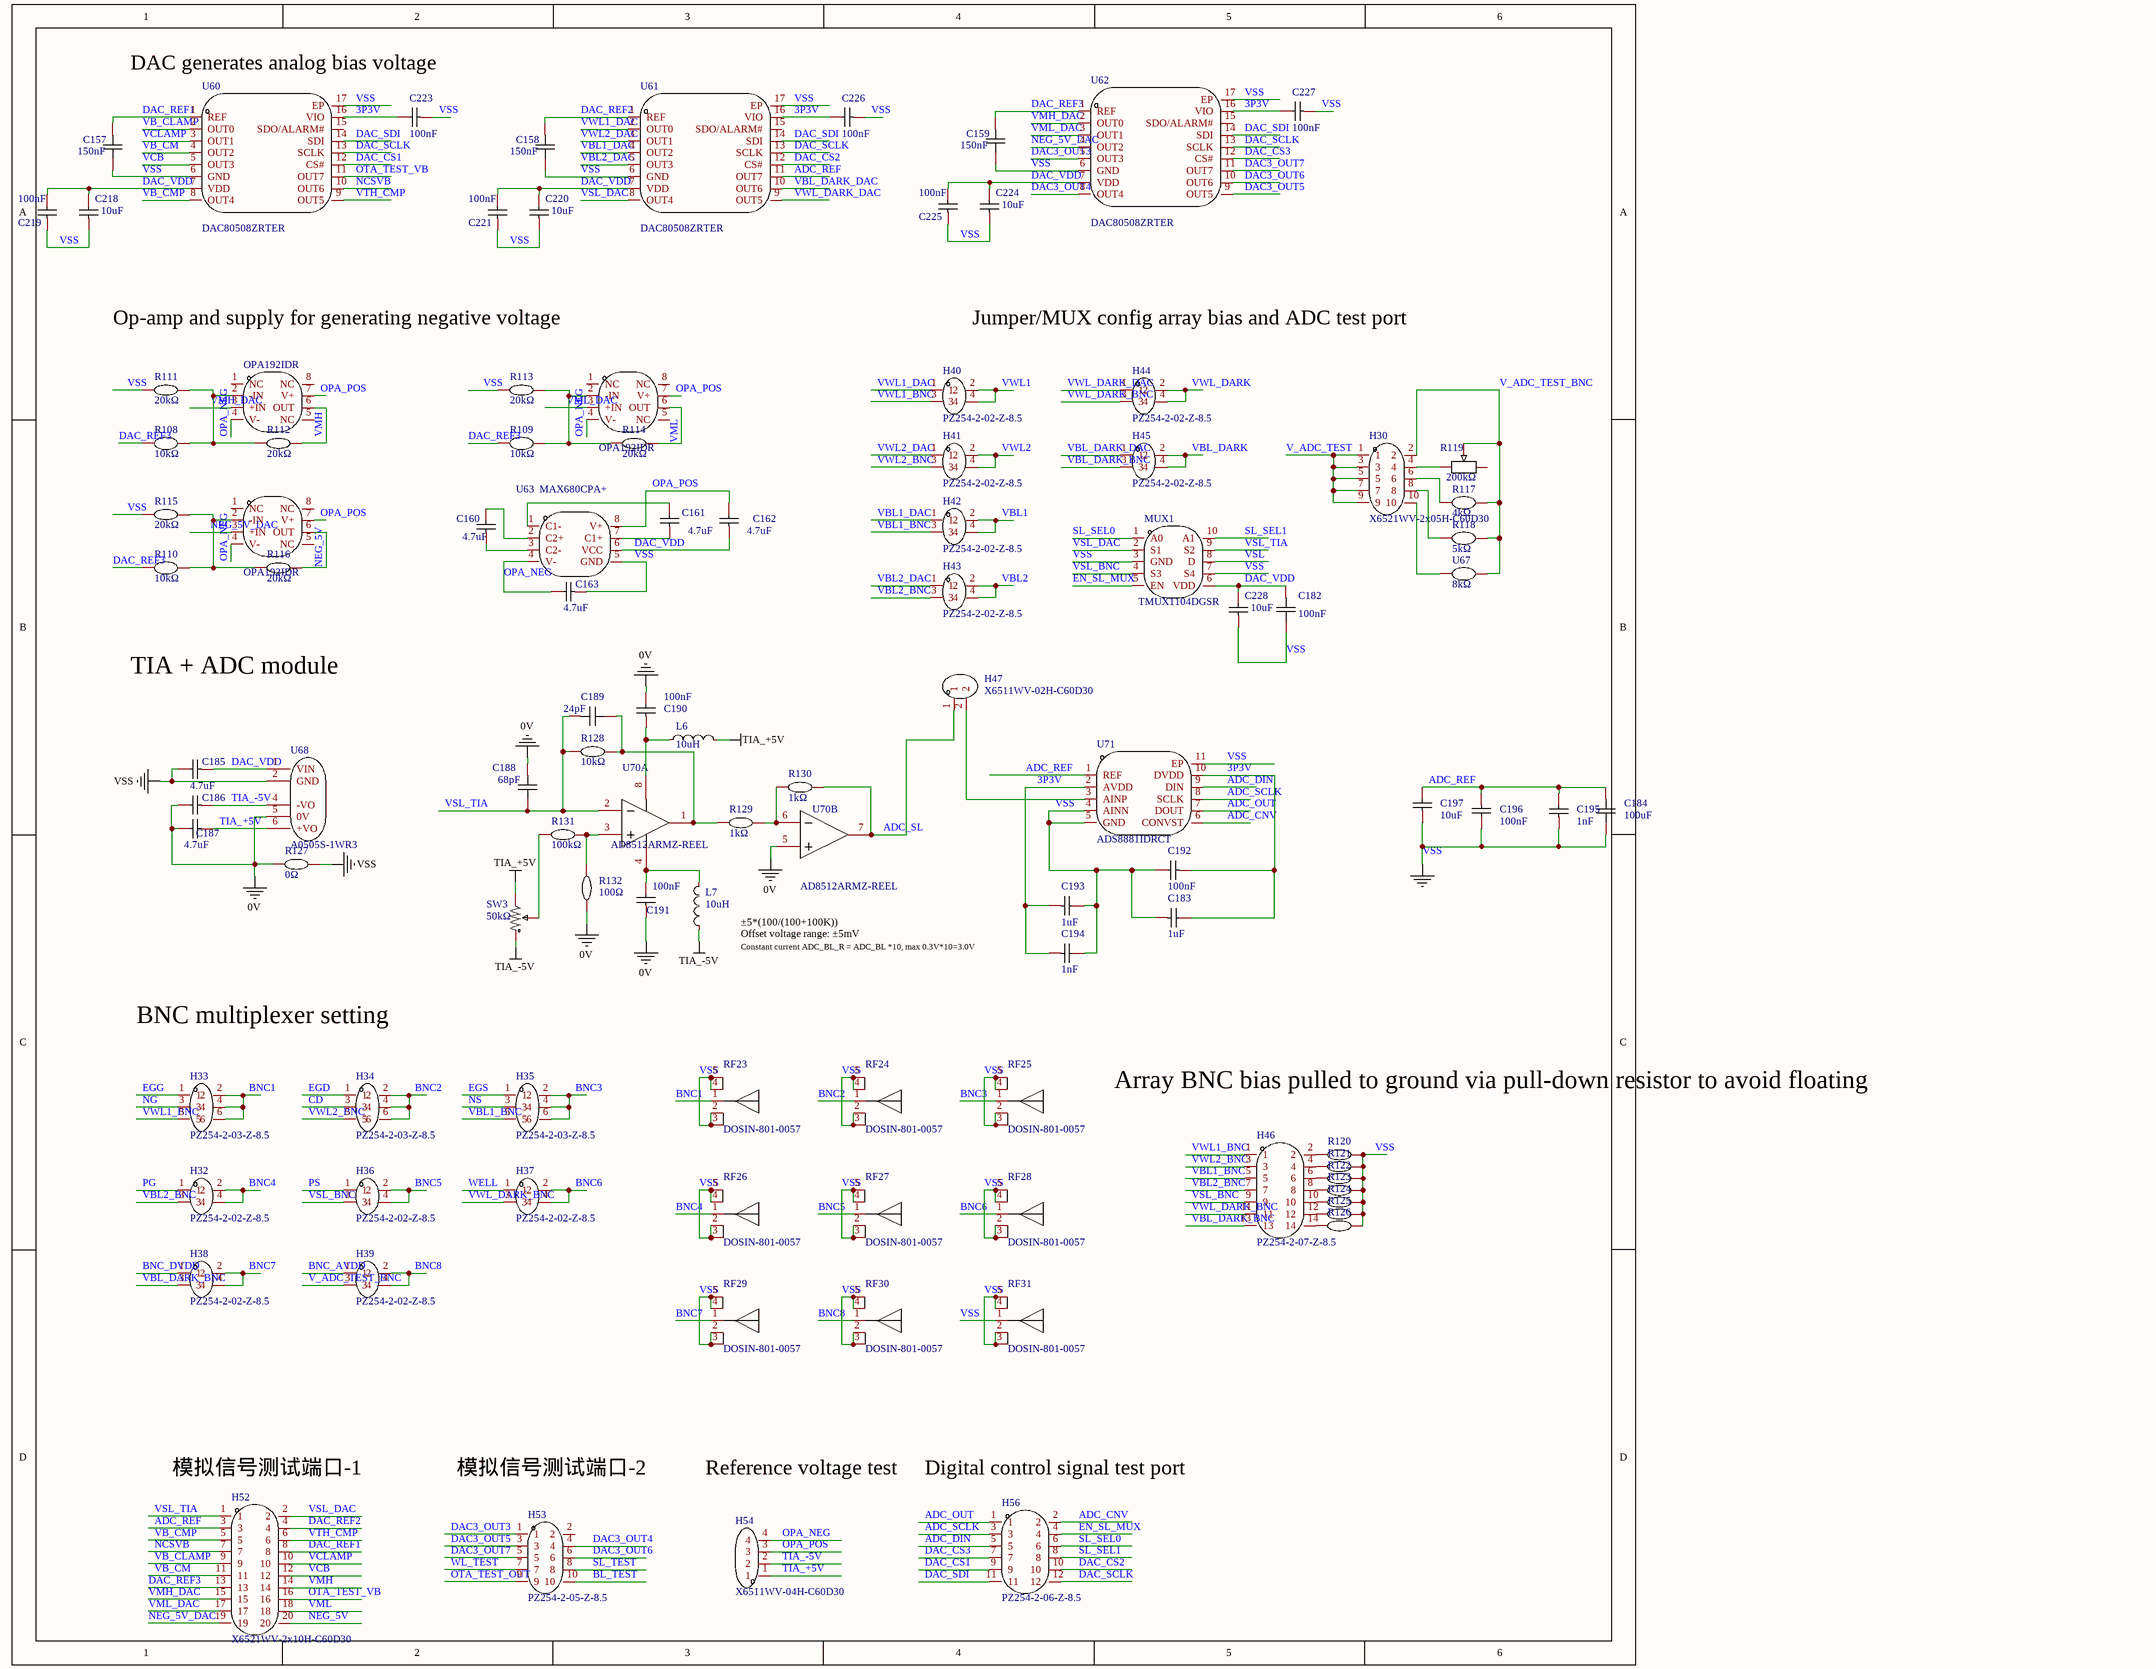
[diagram p0: MISC62793-4.schdoc]
# Altium project MISC62793-14.PrjPcb (part 2 of 4)

## Sheet MISC62793-4.schdoc
size 347 x 355 mm; SheetNumber: 2; SheetTotal: 4

### Parts
C157  150nF  [C0402]
C158  150nF  [C0402]
C159  150nF  [C0402]
C160  4.7uF  [C0805]
C161  4.7uF  [C0805]
C162  4.7uF  [C0805]
C163  4.7uF  [C0805]
C182  100nF  [C0402]
C183  1uF  [C0603]
C184  100uF  [C1210]
C185  4.7uF  [C0805]
C186  4.7uF  [C0805]  (value not drawn)
C187  4.7uF  [C0805]
C188  68pF  [C0402]
C189  24pF  [C0402]
C190  100nF  [C0402]
C191  100nF  [C0402]
C192  100nF  [C0402]
C193  1uF  [C0603]
C194  1nF  [C0603]
C195  1nF  [C0603]
C196  100nF  [C0402]
C197  10uF  [C0805]
C218  10uF  [C0805]
C219  100nF  [C0402]
C220  10uF  [C0805]
C221  100nF  [C0402]
C223  100nF  [C0402]
C224  10uF  [C0805]
C225  100nF  [C0402]
C226  100nF  [C0402]
C227  100nF  [C0402]
C228  10uF  [C0805]
H30  X6521WV-2x05H-C60D30  [HDR-TH_10P-P2.54-V-M-R2-C5-S2.54]
H32  PZ254-2-02-Z-8.5  [HDR-TH_4P-P2.54-V-M-R2-C2-S2.54]
H33  PZ254-2-03-Z-8.5  [HDR-TH_6P-P2.54-V-M-R2-C3-S2.54]
H34  PZ254-2-03-Z-8.5  [HDR-TH_6P-P2.54-V-M-R2-C3-S2.54]
H35  PZ254-2-03-Z-8.5  [HDR-TH_6P-P2.54-V-M-R2-C3-S2.54]
H36  PZ254-2-02-Z-8.5  [HDR-TH_4P-P2.54-V-M-R2-C2-S2.54]
H37  PZ254-2-02-Z-8.5  [HDR-TH_4P-P2.54-V-M-R2-C2-S2.54]
H38  PZ254-2-02-Z-8.5  [HDR-TH_4P-P2.54-V-M-R2-C2-S2.54]
H39  PZ254-2-02-Z-8.5  [HDR-TH_4P-P2.54-V-M-R2-C2-S2.54]
H40  PZ254-2-02-Z-8.5  [HDR-TH_4P-P2.54-V-M-R2-C2-S2.54]
H41  PZ254-2-02-Z-8.5  [HDR-TH_4P-P2.54-V-M-R2-C2-S2.54]
H42  PZ254-2-02-Z-8.5  [HDR-TH_4P-P2.54-V-M-R2-C2-S2.54]
H43  PZ254-2-02-Z-8.5  [HDR-TH_4P-P2.54-V-M-R2-C2-S2.54]
H44  PZ254-2-02-Z-8.5  [HDR-TH_4P-P2.54-V-M-R2-C2-S2.54]
H45  PZ254-2-02-Z-8.5  [HDR-TH_4P-P2.54-V-M-R2-C2-S2.54]
H46  PZ254-2-07-Z-8.5  [HDR-TH_14P-P2.54-V-M-R2-C7-S2.54]
H47  X6511WV-02H-C60D30  [HDR-TH_2P-P2.54-V-M]
H52  X6521WV-2x10H-C60D30  [HDR-TH_20P-P2.54-V-M-R2-C10-S2.54]
H53  PZ254-2-05-Z-8.5  [HDR-TH_10P-P2.54-V-M-R2-C5-S2.54]
H54  X6511WV-04H-C60D30  [HDR-TH_4P-P2.54-V-M]
H56  PZ254-2-06-Z-8.5  [HDR-TH_12P-P2.54-V-M-R2-C6-S2.54]
L6  10uH  [IND-SMD_L7.3-W6.8]
L7  10uH  [IND-SMD_L7.3-W6.8]
MUX1  TMUX1104DGSR  [VSSOP-10_L3.0-W3.0-P0.50-LS4.9-BL]
R108  10kΩ  [R0603]
R109  10kΩ  [R0603]
R110  10kΩ  [R0603]
R111  20kΩ  [R0805]
R112  20kΩ  [R0805]
R113  20kΩ  [R0805]
R114  20kΩ  [R0805]
R115  20kΩ  [R0805]
R116  20kΩ  [R0805]
R117  4kΩ  [R0805]
R118  5kΩ  [R0805]
R119  200kΩ  [RES-ADJ-SMD_3P-L4.5-W4.5-P2.30-BL-FS]
R120  1MΩ  [R1206]  (value not drawn)
R121  1MΩ  [R1206]  (value not drawn)
R122  1MΩ  [R1206]  (value not drawn)
R123  1MΩ  [R1206]  (value not drawn)
R124  1MΩ  [R1206]  (value not drawn)
R125  1MΩ  [R1206]  (value not drawn)
R126  1MΩ  [R1206]  (value not drawn)
R127  0Ω  [R0603]
R128  10kΩ  [R0603]
R129  1kΩ  [R0805]
R130  1kΩ  [R0805]
R131  100kΩ  [R0603]
R132  100Ω  [R1206]
RF23  DOSIN-801-0057  [ANT-TH_DOSIN-801-0057]
RF24  DOSIN-801-0057  [ANT-TH_DOSIN-801-0057]
RF25  DOSIN-801-0057  [ANT-TH_DOSIN-801-0057]
RF26  DOSIN-801-0057  [ANT-TH_DOSIN-801-0057]
RF27  DOSIN-801-0057  [ANT-TH_DOSIN-801-0057]
RF28  DOSIN-801-0057  [ANT-TH_DOSIN-801-0057]
RF29  DOSIN-801-0057  [ANT-TH_DOSIN-801-0057]
RF30  DOSIN-801-0057  [ANT-TH_DOSIN-801-0057]
RF31  DOSIN-801-0057  [ANT-TH_DOSIN-801-0057]
SW3  50kΩ  [RES-ADJ-SMD_3P-L6.0-W4.3-P5.00-BL]
U60  DAC80508ZRTER  [WQFN-16_L3.0-W3.0-P0.50-TL-EP0.8]
U61  DAC80508ZRTER  [WQFN-16_L3.0-W3.0-P0.50-TL-EP0.8]
U62  DAC80508ZRTER  [WQFN-16_L3.0-W3.0-P0.50-TL-EP0.8]
U63  MAX680CPA+  [DIP-8_L10.1-W6.3-P2.54-LS7.6-BL]
U64  OPA192IDR  [SOIC-8_L4.9-W3.9-P1.27-LS6.0-BL]
U65  OPA192IDR  [SOIC-8_L4.9-W3.9-P1.27-LS6.0-BL]
U66  OPA192IDR  [SOIC-8_L4.9-W3.9-P1.27-LS6.0-BL]
U67  8kΩ  [R0805]
U68  A0505S-1WR3  [PWRM-TH_A05XXS-1WR3]
U70  AD8512ARMZ-REEL  [MSOP-8_L3.0-W3.0-P0.65-LS5.0-TL]  (parts A,B of 2)
U71  ADS8881IDRCT  [VSON-10_L3.0-W3.0-P0.50-TL-EP-3]

### Nets
0V: C186.2 C187.2 C188.2 C190.2 C191.1 R127.1 R132.1 U68.5(0V) U70.5(+IN_B)
TIA_+5V: C187.1 H54.1 L6.2 SW3.3 U68.6(+VO)
TIA_-5V: C186.1 H54.2 L7.1 SW3.1 U68.4(-VO)
VSS: C157.1 C158.1 C159.1 C163.1 C182.1 C183.1 C184.1 C185.2 C192.2 C193.2 C194.2 C195.1 C196.2 C197.1 C218.1 C219.1 C220.1 C221.1 C223.1 C224.1 C225.1 C226.1 C227.1 C228.1 MUX1.3(GND) MUX1.7(S4) R111.1 R113.1 R115.1 R120.2 R121.2 R122.2 R123.2 R124.2 R125.2 R126.2 R127.2 RF23.2 RF23.3 RF23.4 RF23.5 RF24.2 RF24.3 RF24.4 RF24.5 RF25.2 RF25.3 RF25.4 RF25.5 RF26.2 RF26.3 RF26.4 RF26.5 RF27.2 RF27.3 RF27.4 RF27.5 RF28.2 RF28.3 RF28.4 RF28.5 RF29.2 RF29.3 RF29.4 RF29.5 RF30.2 RF30.3 RF30.4 RF30.5 RF31.1 RF31.2 RF31.3 RF31.4 RF31.5 U60.6(GND) U60.17(EP) U61.6(GND) U61.17(EP) U62.6(GND) U62.17(EP) U63.5(GND) U68.2(GND) U71.4(AINN) U71.5(GND) U71.11(EP)
3P3V: C183.2 C192.1 C193.1 C194.1 C223.2 C226.2 C227.2 U60.16(VIO) U61.16(VIO) U62.16(VIO) U71.2(AVDD) U71.10(DVDD)
ADC_CNV: H56.2 U71.6(CONVST)
ADC_DIN: H56.5 U71.9(DIN)
ADC_OUT: H56.1 U71.7(DOUT)
ADC_REF: C184.2 C195.2 C196.1 C197.2 H52.3 U61.11(OUT7) U71.1(REF)
ADC_SCLK: H56.3 U71.8(SCLK)
ADC_SL: H47.1 R130.2 U70.7(OUT_B)
BL_TEST: H53.10
BNC1: H33.2 H33.4 H33.6 RF23.1
BNC2: H34.2 H34.4 H34.6 RF24.1
BNC3: H35.2 H35.4 H35.6 RF25.1
BNC4: H32.2 H32.4 RF26.1
BNC5: H36.2 H36.4 RF27.1
BNC6: H37.2 H37.4 RF28.1
BNC7: H38.2 H38.4 RF29.1
BNC8: H39.2 H39.4 RF30.1
BNC_AVDD: H39.1
BNC_DVDD: H38.1
CD: H34.3
DAC3_OUT3: H53.1 U62.5(OUT3)
DAC3_OUT4: H53.4 U62.8(OUT4)
DAC3_OUT5: H53.3 U62.9(OUT5)
DAC3_OUT6: H53.6 U62.10(OUT6)
DAC3_OUT7: H53.5 U62.11(OUT7)
DAC_CS1: H56.9 U60.12(CS#)
DAC_CS2: H56.10 U61.12(CS#)
DAC_CS3: H56.7 U62.12(CS#)
DAC_REF1: C157.2 H52.8 U60.1(REF)
DAC_REF2: C158.2 H52.4 U61.1(REF)
DAC_REF3: C159.2 H52.13 R108.1 R109.1 R110.1 U62.1(REF)
DAC_SCLK: H56.12 U60.13(SCLK) U61.13(SCLK) U62.13(SCLK)
DAC_SDI: H56.11 U60.14(SDI) U61.14(SDI) U62.14(SDI)
DAC_VDD: C162.1 C182.2 C185.1 C218.2 C219.2 C220.2 C221.2 C224.2 C225.2 C228.2 MUX1.6(VDD) U60.7(VDD) U61.7(VDD) U62.7(VDD) U63.6(VCC) U68.1(VIN)
EGD: H34.1
EGG: H33.1
EGS: H35.1
EN_SL_MUX: H56.4 MUX1.5(EN)
NCSVB: H52.7 U60.10(OUT6)
NEG_5V: H52.20 R116.2 U65.6(OUT)
NEG_5V_DAC: H52.19 U62.4(OUT2) U65.3(+IN)
NG: H33.3
NS: H35.3
OPA_NEG: C163.2 H54.4 U63.4(V-) U64.4(V-) U65.4(V-) U66.4(V-)
OPA_POS: C162.2 H54.3 U63.8(V+) U64.7(V+) U65.7(V+) U66.7(V+)
OTA_TEST_OUT: H53.9
OTA_TEST_VB: H52.16 U60.11(OUT7)
PG: H32.1
PS: H36.1
SL_SEL0: H56.6 MUX1.1(A0)
SL_SEL1: H56.8 MUX1.10(A1)
SL_TEST: H53.8
V_ADC_TEST: H30.1 H30.3 H30.5 H30.7 H30.9
V_ADC_TEST_BNC: H30.2 H39.3 R117.2 R118.2 R119.2 U67.2
VB_CLAMP: H52.9 U60.2(OUT0)
VB_CM: H52.11 U60.4(OUT2)
VB_CMP: H52.5 U60.8(OUT4)
VBL1: H42.2 H42.4
VBL1_BNC: H35.5 H42.3 H46.5
VBL1_DAC: H42.1 U61.4(OUT2)
VBL2: H43.2 H43.4
VBL2_BNC: H32.3 H43.3 H46.7
VBL2_DAC: H43.1 U61.5(OUT3)
VBL_DARK: H45.2 H45.4
VBL_DARK_BNC: H38.3 H45.3 H46.13
VBL_DARK_DAC: H45.1 U61.10(OUT6)
VCB: H52.12 U60.5(OUT3)
VCLAMP: H52.10 U60.3(OUT1)
VMH: H52.14 R112.2 U64.6(OUT)
VMH_DAC: H52.15 U62.2(OUT0) U64.3(+IN)
VML: H52.18 R114.2 U66.6(OUT)
VML_DAC: H52.17 U62.3(OUT1) U66.3(+IN)
VSL: MUX1.8(D)
VSL_BNC: H36.3 H46.9 MUX1.4(S3)
VSL_DAC: H52.2 MUX1.2(S1) U61.8(OUT4)
VSL_TIA: C188.1 C189.2 H52.1 MUX1.9(S2) R128.1 U70.2(-IN_A)
VTH_CMP: H52.6 U60.9(OUT5)
VWL1: H40.2 H40.4
VWL1_BNC: H33.5 H40.3 H46.1
VWL1_DAC: H40.1 U61.2(OUT0)
VWL2: H41.2 H41.4
VWL2_BNC: H34.5 H41.3 H46.3
VWL2_DAC: H41.1 U61.3(OUT1)
VWL_DARK: H44.2 H44.4
VWL_DARK_BNC: H37.3 H44.3 H46.11
VWL_DARK_DAC: H44.1 U61.9(OUT5)
WELL: H37.1
WL_TEST: H53.7
NetC160_1: C160.1 U63.3(C2-)
NetC160_2: C160.2 U63.2(C2+)
NetC161_1: C161.1 U63.7(C1+)
NetC161_2: C161.2 U63.1(C1-)
NetC189_1: C189.1 R128.2 R129.1 U70.1(OUT_A)
NetC190_1: C190.1 L6.1 U70.8(V+)
NetC191_2: C191.2 L7.2 U70.4(V-)
NetH30_4: H30.4 R119.1
NetH30_6: H30.6 R117.1
NetH30_8: H30.8 R118.1
NetH30_10: H30.10 U67.1
NetH46_2: H46.2 R120.1
NetH46_4: H46.4 R121.1
NetH46_6: H46.6 R122.1
NetH46_8: H46.8 R123.1
NetH46_10: H46.10 R124.1
NetH46_12: H46.12 R125.1
NetH46_14: H46.14 R126.1
NetH47_2: H47.2 U71.3(AINP)
NetR108_2: R108.2 R111.2 R112.1 U64.2(-IN)
NetR109_2: R109.2 R113.2 R114.1 U66.2(-IN)
NetR110_2: R110.2 R115.2 R116.1 U65.2(-IN)
NetR129_2: R129.2 R130.1 U70.6(-IN_B)
NetR131_1: R131.1 SW3.2
NetR131_2: R131.2 R132.2 U70.3(+IN_A)

Not connected (* = marked no-connect by the designer): H53 2; R119 3; U60 15(SDO/ALARM#); U61 15(SDO/ALARM#); U62 15(SDO/ALARM#); U64 1(NC) 5(NC) 8(NC); U65 1(NC) 5(NC) 8(NC); U66 1(NC) 5(NC) 8(NC)

### Notes on the sheet
- DAC generates analog bias voltage
- Op-amp and supply for generating negative voltage
- Jumper/MUX config array bias and ADC test port
- TIA + ADC module
- (near L7) Offset voltage range: ±5mV
- (near L7) ±5*(100/(100+100K))
- (near L7) Constant current ADC_BL_R = ADC_BL *10, max 0.3V*10=3.0V
- BNC multiplexer setting
- Array BNC bias pulled to ground via pull-down resistor to avoid floating
- (near H52) 模拟信号测试端口-1
- 模拟信号测试端口-2
- Reference voltage test
- (near H56) Digital control signal test port

### Library data of the parts
C157-C159 = CC0402KRX5R7BB154: Manufacturer: YAGEO(国巨); Add into BOM: yes; Tolerance: ±10%; Voltage Rated: 16V; Temperature Coefficient: X5R; Name: 150nF; Symbol: CC0402KRX5R7BB154; Device: CC0402KRX5R7BB154; Supplier: LCSC; Supplier Part: C576725; Manufacturer Part: CC0402KRX5R7BB154; Value: 150nF; JLCPCB Part Class: JLCPCB Part Class: Extended library; LCSC Part Name: 150nF ±10% 16V; Supplier Footprint: 0402; Datasheet: https://example.com/upload/public/pdf/source/20200331/C505498_E84D0E375B576359B11079CF792A6AF0.pdf; Convert to PCB: yes
C160-C163 C185-C187 = CL21A475KBQNNNE: Manufacturer: SAMSUNG(三星); Add into BOM: yes; Tolerance: ±10%; Voltage Rated: 50V; Temperature Coefficient: X5R; Name: 4.7uF; Symbol: CL21A475KBQNNNE; Device: CL21A475KBQNNNE; LCSC Part Name: 4.7uF ±10% 50V; Supplier Part: C98192; Manufacturer Part: CL21A475KBQNNNE; Supplier Footprint: 0805; JLCPCB Part Class: JLCPCB Part Class: Extended library; Datasheet: https://example.com/upload/public/pdf/source/20160218/1457707763339.pdf; Supplier: LCSC; Convert to PCB: yes; Value: 4.7uF
C182 = CC0402KRX7R7BB104: Manufacturer: YAGEO(国巨); Add into BOM: yes; Tolerance: ±10%; Voltage Rated: 16V; Temperature Coefficient: X7R; Name: 100nF; Symbol: CC0402KRX7R7BB104; Device: CC0402KRX7R7BB104; Supplier: LCSC; Manufacturer Part: CC0402KRX7R7BB104; Value: 100nF; Supplier Part: C60474; JLCPCB Part Class: JLCPCB Part Class: Extended library; LCSC Part Name: 100nF ±10% 16V; Supplier Footprint: 0402; Datasheet: https://example.com/upload/public/pdf/source/20211223/9278FD768280B81DDBEF48FA36411A03.pdf; Convert to PCB: yes
C183 C193 = CL10A105KO8NNNC: Manufacturer: SAMSUNG(三星); Add into BOM: yes; Tolerance: ±10%; Voltage Rated: 16V; Temperature Coefficient: X5R; Name: 1uF; Symbol: CL10A105KO8NNNC; Device: CL10A105KO8NNNC; LCSC Part Name: 1uF ±10% 16V; Supplier Part: C1592; Manufacturer Part: CL10A105KO8NNNC; Supplier Footprint: 0603; JLCPCB Part Class: JLCPCB Part Class: Extended library; Datasheet: https://example.com/upload/public/pdf/source/20220919/9FBE606BE0D9532D730F292EB26DC5BB.pdf; Supplier: LCSC; Convert to PCB: yes; Value: 1uF
C184 = EMK325ABJ107MM-P: Manufacturer: TAIYO YUDEN(太诱); Add into BOM: yes; Tolerance: ±20%; Voltage Rated: 16V; Temperature Coefficient: X5R; Name: 100uF; Symbol: EMK325ABJ107MM-P; Device: EMK325ABJ107MM-P; Supplier: LCSC; Supplier Part: C90143; Manufacturer Part: EMK325ABJ107MM-P; Value: 100uF; JLCPCB Part Class: JLCPCB Part Class: Extended library; LCSC Part Name: 100uF ±20% 16V; Supplier Footprint: 1210; Datasheet: https://example.com/upload/public/pdf/source/20190902/C90143_6CB75A095DFF9740D13406046689E055.pdf; Convert to PCB: yes
C188 = CC0402FRNPO9BN680: Manufacturer: YAGEO(国巨); Add into BOM: yes; Tolerance: ±1%; Voltage Rated: 50V; Temperature Coefficient: NP0; Name: 68pF; Symbol: CC0402FRNPO9BN680; Device: CC0402FRNPO9BN680; Supplier: LCSC; Supplier Part: C389103; Manufacturer Part: CC0402FRNPO9BN680; Value: 68pF; JLCPCB Part Class: JLCPCB Part Class: Extended library; LCSC Part Name: 68pF ±1% 50V; Supplier Footprint: 0402; Datasheet: https://example.com/upload/public/pdf/source/20190423/C389103_68497E1D404C7FF179120BC230675ADA.pdf; Convert to PCB: yes
C189 = GJM1555C1H240FB01D: Manufacturer: muRata(村田); Add into BOM: yes; Tolerance: ±1%; Voltage Rated: 50V; Temperature Coefficient: C0G; Name: 24pF; Symbol: GJM1555C1H240FB01D; Device: GJM1555C1H240FB01D; Supplier: LCSC; Supplier Part: C415394; Manufacturer Part: GJM1555C1H240FB01D; Value: 24pF; JLCPCB Part Class: JLCPCB Part Class: Extended library; LCSC Part Name: 24pF ±1% 50V; Supplier Footprint: 0402; Datasheet: https://example.com/upload/public/pdf/source/20190904/C426118_85E81C7C1F21FC87C5FB6D536E0847B4.pdf; Convert to PCB: yes
C190-C192 C196 C219 C221 C223 C225-C227 = CL05B104KO5NNNC: Manufacturer: SAMSUNG(三星); Add into BOM: yes; Tolerance: ±10%; Voltage Rated: 16V; Temperature Coefficient: X7R; Name: 100nF; Symbol: CL05B104KO5NNNC; Device: CL05B104KO5NNNC; Supplier: LCSC; Manufacturer Part: CL05B104KO5NNNC; Value: 100nF; Supplier Part: C1525; JLCPCB Part Class: JLCPCB Part Class: Basic library; LCSC Part Name: 100nF ±10% 16V; Supplier Footprint: 0402; Datasheet: https://example.com/upload/public/pdf/source/20160218/1457707763339.pdf; Convert to PCB: yes
C194 C195 = CC0603KRX7R9BB102: Manufacturer: YAGEO(国巨); Add into BOM: yes; Tolerance: ±10%; Voltage Rated: 50V; Temperature Coefficient: X7R; Name: 1nF; Symbol: CC0603KRX7R9BB102; Device: CC0603KRX7R9BB102; Supplier: LCSC; Manufacturer Part: CC0603KRX7R9BB102; Value: 1nF; Supplier Part: C100040; JLCPCB Part Class: JLCPCB Part Class: Extended library; LCSC Part Name: 1nF ±10% 50V; Supplier Footprint: 0603; Datasheet: https://example.com/upload/public/pdf/source/20180910/C282072_33301C7F631E79921B82A8DAC6BCC5B3.pdf; Convert to PCB: yes
C197 C218 C220 C224 C228 = CL21A106KOQNNNE: Manufacturer: SAMSUNG(三星); Add into BOM: yes; Tolerance: ±10%; Voltage Rated: 16V; Temperature Coefficient: X5R; Name: 10uF; Symbol: CL21A106KOQNNNE; Device: CL21A106KOQNNNE; Supplier: LCSC; Manufacturer Part: CL21A106KOQNNNE; Value: 10uF; Supplier Part: C1713; JLCPCB Part Class: JLCPCB Part Class: Extended library; LCSC Part Name: 10uF ±10% 16V; Supplier Footprint: 0805; Datasheet: https://example.com/upload/public/pdf/source/20160218/1457707763339.pdf; Convert to PCB: yes
H30 = X6521WV-2x05H-C60D30: Manufacturer: XKB Connection(中国星坤); Symbol: X6521WV-2×05H-C30D60; Add into BOM: yes; Pin Structure: 2x5P; Pitch: 2.54mm; Circluar Pins/Square Pins: Square pin; Current Rating (Max): 3A; Voltage Rating (Max): 250V; Soldering Temperature(Max): 260℃; Name: X6521WV-2x05H-C60D30; Device: X6521WV-2x05H-C60D30; LCSC Part Name: 2x5P 间距:2.54mm 方针; Supplier Part: C706895; Manufacturer Part: X6521WV-2x05H-C60D30; Supplier Footprint: 插件,P=2.54mm; JLCPCB Part Class: JLCPCB Part Class: Extended library; Datasheet: https://example.com/upload/public/pdf/source/20211009/DE33EBA4104B5B447A7BD8383FBBA145.pdf; Supplier: LCSC; Convert to PCB: yes; Row Spacing: 2.54mm; Mounting Type: -; Number of Rows: Dual row; Number of Pins: 10P; Length of Mating Pin: 6mm; Insulation Height: 2.5mm; Length of End Connection Pin: 3mm; Contact Material: Brass; Contact Plating: Gold; Operating Temperature Range: -40℃~+105℃; Color: Black
H32 H36-H45 = PZ254-2-02-Z-8.5_C2894963: Manufacturer: HCTL(华灿天禄); Add into BOM: yes; Pin Structure: 2x2P; Pitch: 2.54mm; Circluar Pins/Square Pins: Square pin; Current Rating (Max): 3A; Soldering Temperature(Max): 260℃@10S; Name: PZ254-2-02-Z-8.5; Symbol: PZ254-2-02-Z-8.5; Device: PZ254-2-02-Z-8.5_C2894963; LCSC Part Name: 2x2P 间距:2.54mm 方针 直插; Supplier Part: C2894963; Manufacturer Part: PZ254-2-02-Z-8.5; Supplier Footprint: 插件,P=2.54mm; JLCPCB Part Class: JLCPCB Part Class: Extended library; Datasheet: https://example.com/upload/public/pdf/source/20230609/5BA09C8BEB9B31376F8BF6032FF67CAC.pdf; Supplier: LCSC; Convert to PCB: yes; Row Spacing: 2.54mm; Mounting Type: Through hole; Number of Rows: Dual row; Number of Pins: 4P; Voltage Rating (Max): -; Length of Mating Pin: 6mm; Insulation Height: 2.5mm; Length of End Connection Pin: 3mm; Contact Material: Brass; Operating Temperature Range: -40℃~+105℃; Color: Black
H33-H35 = PZ254-2-03-Z-8.5_C2894964: Manufacturer: HCTL(华灿天禄); Add into BOM: yes; Pin Structure: 2x3P; Pitch: 2.54mm; Circluar Pins/Square Pins: Square pin; Current Rating (Max): 3A; Soldering Temperature(Max): 260℃@10S; Name: PZ254-2-03-Z-8.5; Symbol: PZ254-2-03-Z-8.5; Device: PZ254-2-03-Z-8.5_C2894964; LCSC Part Name: 2x3P 间距:2.54mm 方针 直插; Supplier Part: C2894964; Manufacturer Part: PZ254-2-03-Z-8.5; Supplier Footprint: 插件,P=2.54mm; JLCPCB Part Class: JLCPCB Part Class: Extended library; Datasheet: https://example.com/upload/public/pdf/source/20230609/5BA09C8BEB9B31376F8BF6032FF67CAC.pdf; Supplier: LCSC; Convert to PCB: yes; Row Spacing: 2.54mm; Mounting Type: Through hole; Number of Rows: Dual row; Number of Pins: 6P; Voltage Rating (Max): -; Length of Mating Pin: 6mm; Insulation Height: 2.5mm; Length of End Connection Pin: 3mm; Contact Material: Brass; Operating Temperature Range: -40℃~+105℃; Color: Black
H46 = PZ254-2-07-Z-8.5: Manufacturer: HCTL(华灿天禄); Add into BOM: yes; Pin Structure: 2x7P; Pitch: 2.54mm; Circluar Pins/Square Pins: Square pin; Current Rating (Max): 3A; Soldering Temperature(Max): 260℃@10S; Name: PZ254-2-07-Z-8.5; Symbol: PZ254-2-07-Z-8.5; Device: PZ254-2-07-Z-8.5; LCSC Part Name: 2x7P 间距:2.54mm 方针 直插; Supplier Part: C2894968; Manufacturer Part: PZ254-2-07-Z-8.5; Supplier Footprint: 插件,P=2.54mm; JLCPCB Part Class: JLCPCB Part Class: Extended library; Datasheet: https://example.com/upload/public/pdf/source/20230609/5BA09C8BEB9B31376F8BF6032FF67CAC.pdf; Supplier: LCSC; Convert to PCB: yes; Row Spacing: 2.54mm; Mounting Type: Through hole; Number of Rows: Dual row; Number of Pins: 14P; Voltage Rating (Max): -; Length of Mating Pin: 6mm; Insulation Height: 2.5mm; Length of End Connection Pin: 3mm; Contact Material: Brass; Operating Temperature Range: -40℃~+105℃; Color: Black
H47 = X6511WV-02H-C60D30: Manufacturer: XKB Connection(中国星坤); Symbol: X6511WV-02H-C30D60; Add into BOM: yes; Pin Structure: 1x2P; Pitch: 2.54mm; Circluar Pins/Square Pins: Square pin; Current Rating (Max): 3A; Voltage Rating (Max): 250V; Soldering Temperature(Max): 260℃; Name: X6511WV-02H-C60D30; Device: X6511WV-02H-C60D30; LCSC Part Name: 1x2P 间距:2.54mm 方针; Supplier Part: C706874; Manufacturer Part: X6511WV-02H-C60D30; Supplier Footprint: 插件,P=2.54mm; JLCPCB Part Class: JLCPCB Part Class: Extended library; Supplier: LCSC; Convert to PCB: yes; Row Spacing: 2.54mm; Mounting Type: -; Number of Rows: Single row; Number of Pins: 2P; Length of Mating Pin: 6mm; Insulation Height: 2.5mm; Length of End Connection Pin: 3mm; Contact Material: Brass; Contact Plating: Gold; Operating Temperature Range: -40℃~+105℃; Color: Black
H52 = X6521WV-2x10H-C60D30: Manufacturer: XKB Connection(中国星坤); Symbol: X6521WV-2×10H-C30D60; Add into BOM: yes; Pin Structure: 2x10P; Pitch: 2.54mm; Circluar Pins/Square Pins: Square pin; Current Rating (Max): 3A; Voltage Rating (Max): 250V; Soldering Temperature(Max): 260℃; Name: X6521WV-2x10H-C60D30; Device: X6521WV-2x10H-C60D30; LCSC Part Name: 2x10P 间距:2.54mm 方针; Supplier Part: C706900; Manufacturer Part: X6521WV-2x10H-C60D30; Supplier Footprint: 插件,P=2.54mm; JLCPCB Part Class: JLCPCB Part Class: Extended library; Datasheet: https://example.com/upload/public/pdf/source/20211009/DE33EBA4104B5B447A7BD8383FBBA145.pdf; Supplier: LCSC; Convert to PCB: yes; Row Spacing: 2.54mm; Mounting Type: -; Number of Rows: Dual row; Number of Pins: 20P; Length of Mating Pin: 6mm; Insulation Height: 2.5mm; Length of End Connection Pin: 3mm; Contact Material: Brass; Contact Plating: Gold; Operating Temperature Range: -40℃~+105℃; Color: Black
H53 = PZ254-2-05-Z-8.5_C2894966: Manufacturer: HCTL(华灿天禄); Add into BOM: yes; Pin Structure: 2x5P; Pitch: 2.54mm; Circluar Pins/Square Pins: Square pin; Current Rating (Max): 3A; Soldering Temperature(Max): 260℃@10S; Name: PZ254-2-05-Z-8.5; Symbol: PZ254-2-05-Z-8.5; Device: PZ254-2-05-Z-8.5_C2894966; LCSC Part Name: 2x5P 间距:2.54mm 方针 直插; Supplier Part: C2894966; Manufacturer Part: PZ254-2-05-Z-8.5; Supplier Footprint: 插件,P=2.54mm; JLCPCB Part Class: JLCPCB Part Class: Extended library; Datasheet: https://example.com/upload/public/pdf/source/20230609/5BA09C8BEB9B31376F8BF6032FF67CAC.pdf; Supplier: LCSC; Convert to PCB: yes; Row Spacing: 2.54mm; Mounting Type: Through hole; Number of Rows: Dual row; Number of Pins: 10P; Voltage Rating (Max): -; Length of Mating Pin: 6mm; Insulation Height: 2.5mm; Length of End Connection Pin: 3mm; Contact Material: Brass; Operating Temperature Range: -40℃~+105℃; Color: Black
H54 = X6511WV-04H-C60D30: Manufacturer: XKB Connection(中国星坤); Symbol: X6511WV-04H-C30D60; Add into BOM: yes; Pin Structure: 1x4P; Pitch: 2.54mm; Circluar Pins/Square Pins: Square pin; Current Rating (Max): 3A; Voltage Rating (Max): 250V; Soldering Temperature(Max): 260℃; Name: X6511WV-04H-C60D30; Device: X6511WV-04H-C60D30; LCSC Part Name: 1x4P 间距:2.54mm 方针; Supplier Part: C706876; Manufacturer Part: X6511WV-04H-C60D30; Supplier Footprint: 插件,P=2.54mm; JLCPCB Part Class: JLCPCB Part Class: Extended library; Datasheet: https://example.com/upload/public/pdf/source/20211009/D19569EFFEB9776B42364DF7D41FD96A.pdf; Supplier: LCSC; Convert to PCB: yes; Row Spacing: 2.54mm; Mounting Type: -; Number of Rows: Single row; Number of Pins: 4P; Length of Mating Pin: 6mm; Insulation Height: 2.5mm; Length of End Connection Pin: 3mm; Contact Material: Brass; Contact Plating: Gold; Operating Temperature Range: -40℃~+105℃; Color: Black
H56 = PZ254-2-06-Z-8.5: Manufacturer: HCTL(华灿天禄); Add into BOM: yes; Pin Structure: 2x6P; Pitch: 2.54mm; Circluar Pins/Square Pins: Square pin; Current Rating (Max): 3A; Soldering Temperature(Max): 260℃@10S; Name: PZ254-2-06-Z-8.5; Symbol: PZ254-2-06-Z-8.5; Device: PZ254-2-06-Z-8.5; LCSC Part Name: 2x6P 间距:2.54mm 方针 直插; Supplier Part: C2894967; Manufacturer Part: PZ254-2-06-Z-8.5; Supplier Footprint: 插件,P=2.54mm; JLCPCB Part Class: JLCPCB Part Class: Extended library; Datasheet: https://example.com/upload/public/pdf/source/20230609/5BA09C8BEB9B31376F8BF6032FF67CAC.pdf; Supplier: LCSC; Convert to PCB: yes; Row Spacing: 2.54mm; Mounting Type: Through hole; Number of Rows: Dual row; Number of Pins: 12P; Voltage Rating (Max): -; Length of Mating Pin: 6mm; Insulation Height: 2.5mm; Length of End Connection Pin: 3mm; Contact Material: Brass; Operating Temperature Range: -40℃~+105℃; Color: Black
L6 L7 = FXL0630-100-M: Manufacturer: cjiang(长江微电); Add into BOM: yes; Tolerance: ±20%; Rated Current: 4.5A; Saturation Current (Isat): 5.5A; DC Resistance (DCR): 68mΩ; Type: Molded inductor; Name: 10uH; Symbol: FXL0630-100-M; Device: FXL0630-100-M; LCSC Part Name: 10uH ±20% 5.5A; Supplier Part: C167223; Manufacturer Part: FXL0630-100-M; Supplier Footprint: SMD,6.6x7mm; JLCPCB Part Class: JLCPCB Part Class: Extended library; Datasheet: https://example.com/upload/public/pdf/source/20230516/3A080F5AF8C87BB81C3BA86E5F60E51A.pdf; Supplier: LCSC; Convert to PCB: yes; Value: 10uH; Ratings: -
MUX1 = TMUX1104DGSR: Manufacturer: TI(德州仪器); Add into BOM: yes; Switch Circuit: SP4T; Number of Channels: 1; Turn-on time: 12ns; On-State Resistance (Max): 4Ω; Turn-off time: 5ns; Name: TMUX1104DGSR; Symbol: TMUX1104DGSR; Device: TMUX1104DGSR; LCSC Part Name: TMUX1104DGSR; Supplier Part: C2879206; Manufacturer Part: TMUX1104DGSR; Supplier Footprint: MSOP-10; JLCPCB Part Class: JLCPCB Part Class: Extended library; Supplier: LCSC; Convert to PCB: yes